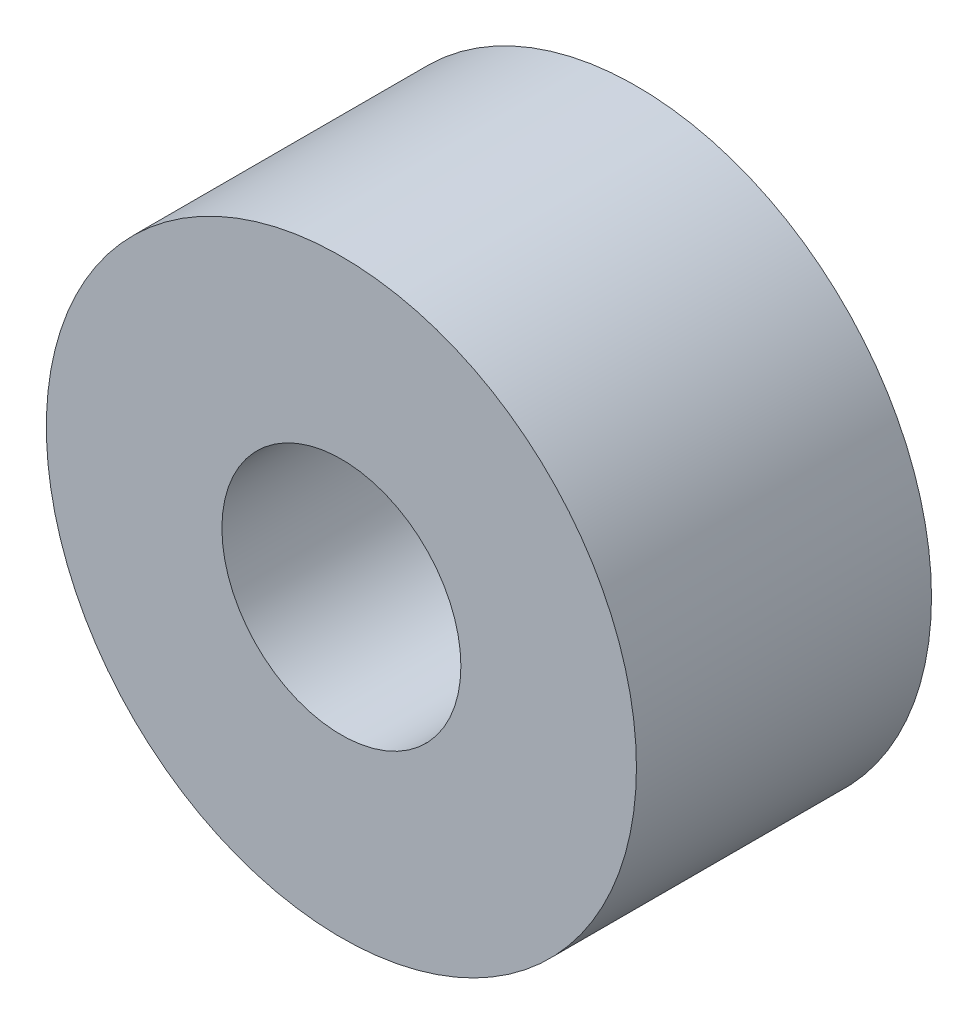
SolidWorks part; units mm, degrees
ref_plane "前视基准面" through (0, 0, 0) normal (0, 0, 1) x (1, 0, 0)
ref_plane "上视基准面" through (0, 0, 0) normal (0, 1, 0) x (1, 0, 0)
ref_plane "右视基准面" through (0, 0, 0) normal (1, 0, 0) x (0, 0, -1)
other "Configuration Table"
sketch "草图1" plane through (0, 0, 0) normal (0, 0, 1) x (1, 0, 0)
  circle A0 centre (0, 0) radius 20
  circle A1 centre (0, 0) radius 8.1
  point P0 (0, 0)
  dimension "D1" = 16.2
  dimension "D2" = 40
extrude "凸台-拉伸1" add sketch "草图1" against normal mid plane 20
